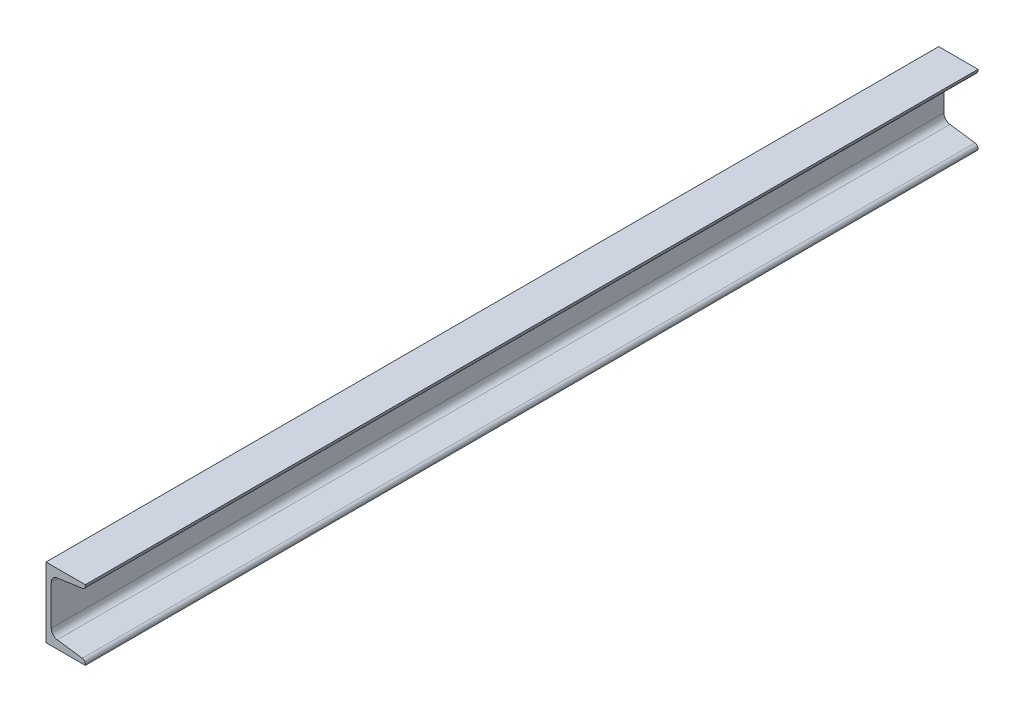
SolidWorks part; units mm, degrees
material "1023 碳钢板 (SS)"
ref_plane "Front Plane" through (0, 0, 0) normal (0, 0, 1) x (1, 0, 0)
ref_plane "Top Plane" through (0, 0, 0) normal (0, 1, 0) x (1, 0, 0)
ref_plane "Right Plane" through (0, 0, 0) normal (1, 0, 0) x (0, 0, -1)
sketch "Sketch1" plane through (0, 0, 0) normal (0, 0, 1) x (1, 0, 0)
  line L0 (0, 0) -> (-45, 0)
  line L1 (-45, 0) -> (-45, -80)
  line L2 (-45, -80) -> (0, -80)
  line L3 (0, -80) -> (0, -78.6393)
  line L4 (-3.4433, -74.6782) -> (-32.1134, -70.6489)
  line L5 (-39, -62.7268) -> (-39, -17.2732)
  line L6 (-32.1134, -9.3511) -> (-3.4433, -5.3218)
  line L7 (0, -1.3607) -> (0, 0)
  line L8 (-22.5, -72) -> (-22.5, -80) construction
  arc A0 (-39, -17.2732) -> (-32.1134, -9.3511) centre (-31, -17.2732) cw
  arc A1 (-32.1134, -70.6489) -> (-39, -62.7268) centre (-31, -62.7268) cw
  arc A2 (-3.4433, -5.3218) -> (0, -1.3607) centre (-4, -1.3607) ccw
  arc A3 (0, -78.6393) -> (-3.4433, -74.6782) centre (-4, -78.6393) ccw
  dimension "D8" = 8
  dimension "D9" = 4
  dimension "D1" = 80
  dimension "D2" = 45
  dimension "D3" = 6
  dimension "D4" = 22.5
  dimension "D5" = 8
  dimension "D6" = 8
  dimension "D7" = 8
extrude "Boss-Extrude1" add sketch "Sketch1" along normal blind 1022 contours L7 L0 L1 L2 L3 A3 L4 A1 L5 A0 L6 A2
